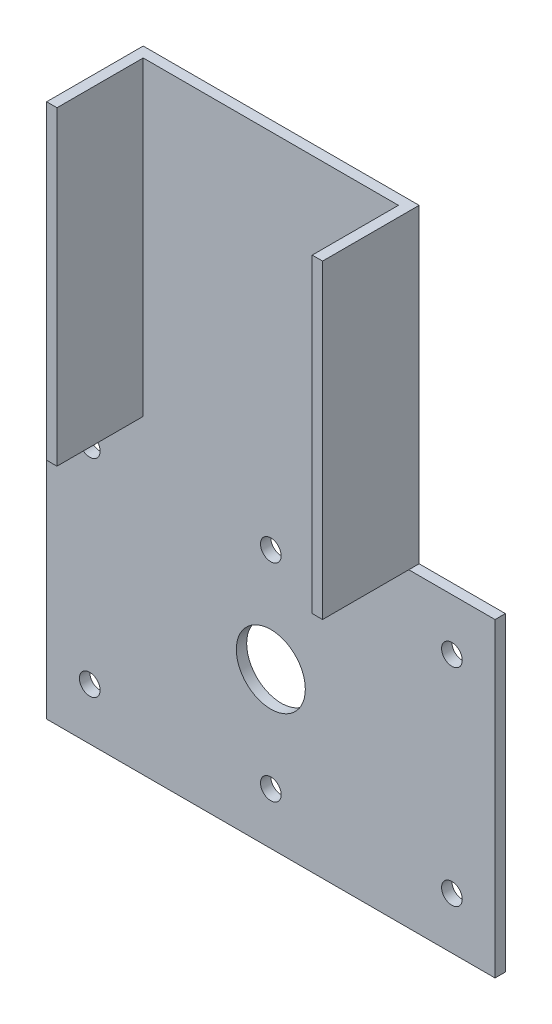
SolidWorks part; units mm, degrees
ref_plane "前视基准面" through (0, 0, 0) normal (0, 0, 1) x (1, 0, 0)
ref_plane "上视基准面" through (0, 0, 0) normal (0, 1, 0) x (1, 0, 0)
ref_plane "右视基准面" through (0, 0, 0) normal (1, 0, 0) x (0, 0, -1)
sketch "草图1" plane through (0, 0, 0) normal (0, 0, 1) x (1, 0, 0)
  line L0 (0, 0) -> (-130, 0)
  line L1 (-130, 0) -> (-130, 90)
  line L2 (-105, 180) -> (-25, 180)
  line L3 (0, 90) -> (0, 0)
  line L4 (0, 90) -> (-130, 90)
  line L6 (-25, 180) -> (-25, 90)
  line L8 (-105, 180) -> (-105, 90)
extrude "凸台-拉伸1" add sketch "草图1" along normal blind 3 contours L2 L8 L4 L6 | L3 L4 L1 L0
sketch "草图2" plane through (0, 0, 3) normal (0, 0, 1) x (1, 0, 0)
  line L0 (-105, 180) -> (-105, 90)
  line L1 (-25, 180) -> (-25, 90)
  line L2 (-102, 180) -> (-102, 90)
  line L3 (-28, 180) -> (-28, 90)
  line L4 (-105, 180) -> (-102, 180)
  line L5 (-105, 90) -> (-102, 90)
  line L6 (-28, 90) -> (-25, 90)
  line L7 (-28, 180) -> (-25, 180)
  dimension "D1" = 3
  dimension "D2" = 3
extrude "凸台-拉伸2" add sketch "草图2" along normal blind 25
sketch "草图3" plane through (0, 0, 0) normal (0, 0, -1) x (-1, 0, 0)
  circle A0 centre (65, 45) radius 10
  circle A1 centre (12.5, 15) radius 3
  circle A2 centre (65, 15) radius 3
  circle A3 centre (117.5, 15) radius 3
  circle A4 centre (117.5, 75) radius 3
  circle A5 centre (65, 75) radius 3
  circle A6 centre (12.5, 75) radius 3
extrude "切除-拉伸1" cut sketch "草图3" against normal blind 25
